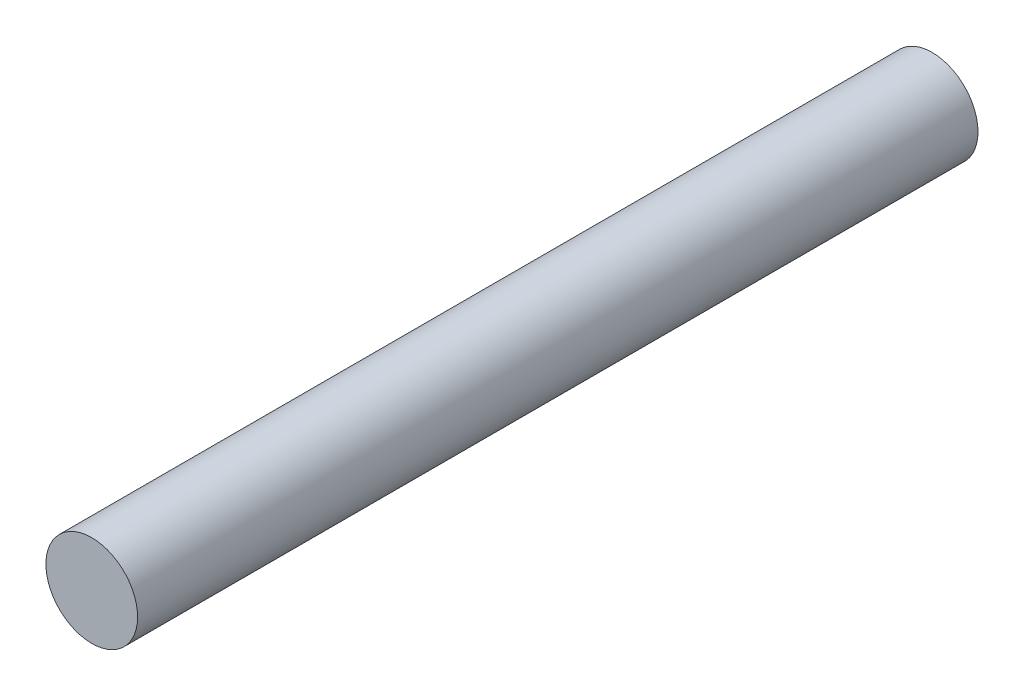
SolidWorks part; units mm, degrees
ref_plane "前视基准面" through (0, 0, 0) normal (0, 0, 1) x (1, 0, 0)
ref_plane "上视基准面" through (0, 0, 0) normal (0, 1, 0) x (1, 0, 0)
ref_plane "右视基准面" through (0, 0, 0) normal (1, 0, 0) x (0, 0, -1)
sketch "草图1" plane through (0, 0, 0) normal (0, 0, 1) x (1, 0, 0)
  circle A0 centre (0, 0) radius 3
  dimension "D1" = 6
extrude "凸台-拉伸2" add sketch "草图1" along normal blind 55
cosmetic thread "装饰螺纹线2" parameters "D2"=5
